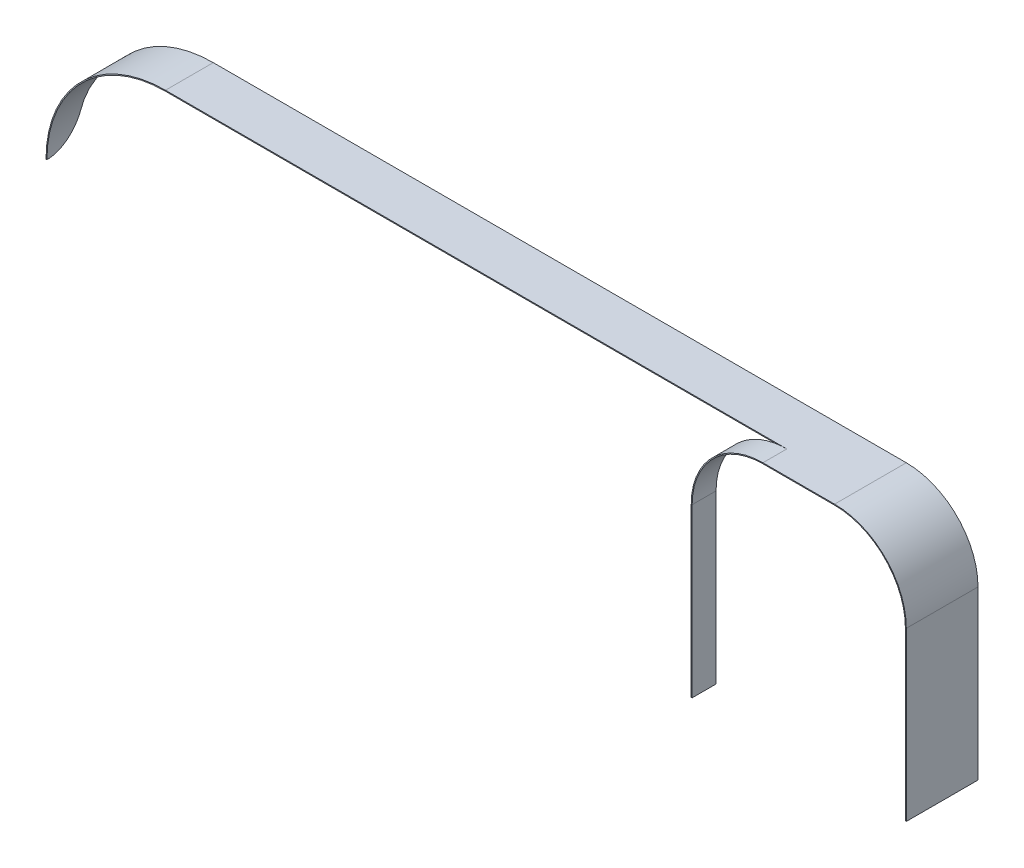
from build123d import *

# Parameters (mm, degrees)
BOSS_EXTRUDE1_DEPTH = 101.6
BOSS_EXTRUDE2_START = 50.8
BOSS_EXTRUDE2_DEPTH = 50.8
CUT_EXTRUDE1_DEPTH  = 800


with BuildPart() as part:
    # Sketch1 → Boss-Extrude1 (new body)
    with BuildSketch(Plane.XY):
        with BuildLine():
            Line((0, 254), (1473.2, 254))
            ThreePointArc((1473.2, 254), (1580.963073453, 209.363073453), (1625.6, 101.6))
            Line((1625.6, 101.6), (1625.6, -254))
            Line((1625.6, -254), (1623.6, -254))
            Line((1623.6, -254), (1623.6, 101.6))
            ThreePointArc((1623.6, 101.6), (1579.54885989, 207.94885989), (1473.2, 252))
            Line((1473.2, 252), (0, 252))
            ThreePointArc((0, 252), (-178.190908859, 178.190908859), (-252, 0))
            Line((-252, 0), (-254, 0))
            ThreePointArc((-254, 0), (-179.605122421, 179.605122421), (0, 254))
        make_face()
    extrude(amount=-BOSS_EXTRUDE1_DEPTH)

    # Sketch2 → Boss-Extrude2 (add)
    with BuildSketch(Plane.XY.offset(BOSS_EXTRUDE2_START)):
        with BuildLine():
            Line((1625.6, -254), (1625.6, 101.6))
            ThreePointArc((1625.6, 101.6), (1580.963073453, 209.363073453), (1473.2, 254))
            Line((1473.2, 254), (1320.8, 254))
            ThreePointArc((1320.8, 254), (1213.036926547, 209.363073453), (1168.4, 101.6))
            Line((1168.4, 101.6), (1168.4, -254))
            Line((1168.4, -254), (1170.4, -254))
            Line((1170.4, -254), (1170.4, 101.6))
            ThreePointArc((1170.4, 101.6), (1214.45114011, 207.94885989), (1320.8, 252))
            Line((1320.8, 252), (1473.2, 252))
            ThreePointArc((1473.2, 252), (1579.54885989, 207.94885989), (1623.6, 101.6))
            Line((1623.6, 101.6), (1623.6, -254))
            Line((1623.6, -254), (1625.6, -254))
        make_face()
    extrude(amount=-BOSS_EXTRUDE2_DEPTH)

    # Sketch3 → Cut-Extrude1 (cut)
    with BuildSketch(Plane(origin=(0, 0, 0), x_dir=(0, 0, -1), z_dir=(1, 0, 0))):
        with BuildLine():
            Line((101.6, 172.72), (101.6, 0))
            Line((101.6, 0), (0, 0))
            ThreePointArc((0, 0), (44.901280605, 18.598719395), (63.5, 63.5))
            Line((63.5, 63.5), (63.5, 134.62))
            ThreePointArc((63.5, 134.62), (74.659231637, 161.560768363), (101.6, 172.72))
        make_face()
    extrude(amount=-CUT_EXTRUDE1_DEPTH, mode=Mode.SUBTRACT)


solid = part.part
